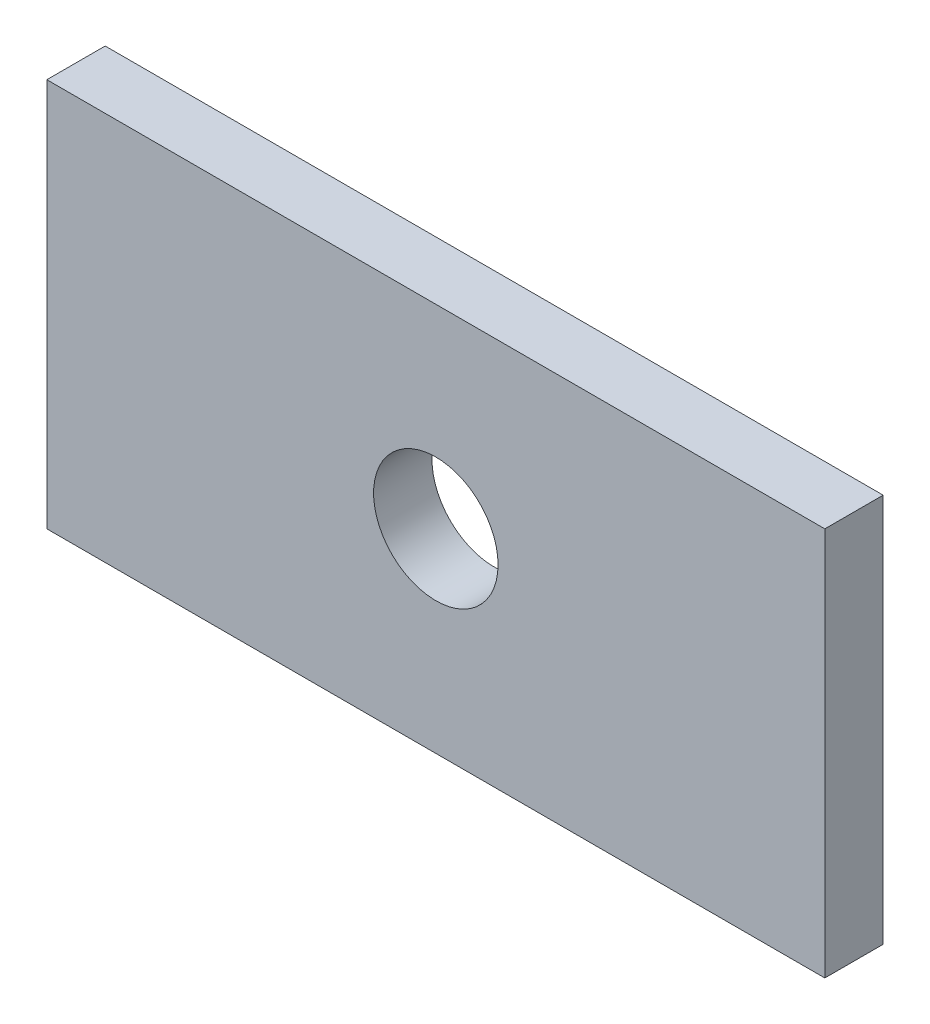
from build123d import *

# Parameters (mm, degrees)
SKETCH_1_W          = 40
SKETCH_1_H          = 20
EXTRUDE_1_DEPTH     = 1.5
SKETCH_2_R          = 3.2
CUT_EXTRUDE_1_DEPTH = 11.5


with BuildPart() as part:
    # 草图1 → 凸台-拉伸1 (new, symmetric)
    with BuildSketch(Plane.XY):
        Rectangle(SKETCH_1_W, SKETCH_1_H)
    extrude(amount=EXTRUDE_1_DEPTH, both=True)

    # 草图2 → 切除-拉伸1 (cut, symmetric)
    with BuildSketch(Plane.XY):
        Circle(SKETCH_2_R)
    extrude(amount=CUT_EXTRUDE_1_DEPTH, both=True, mode=Mode.SUBTRACT)


solid = part.part
